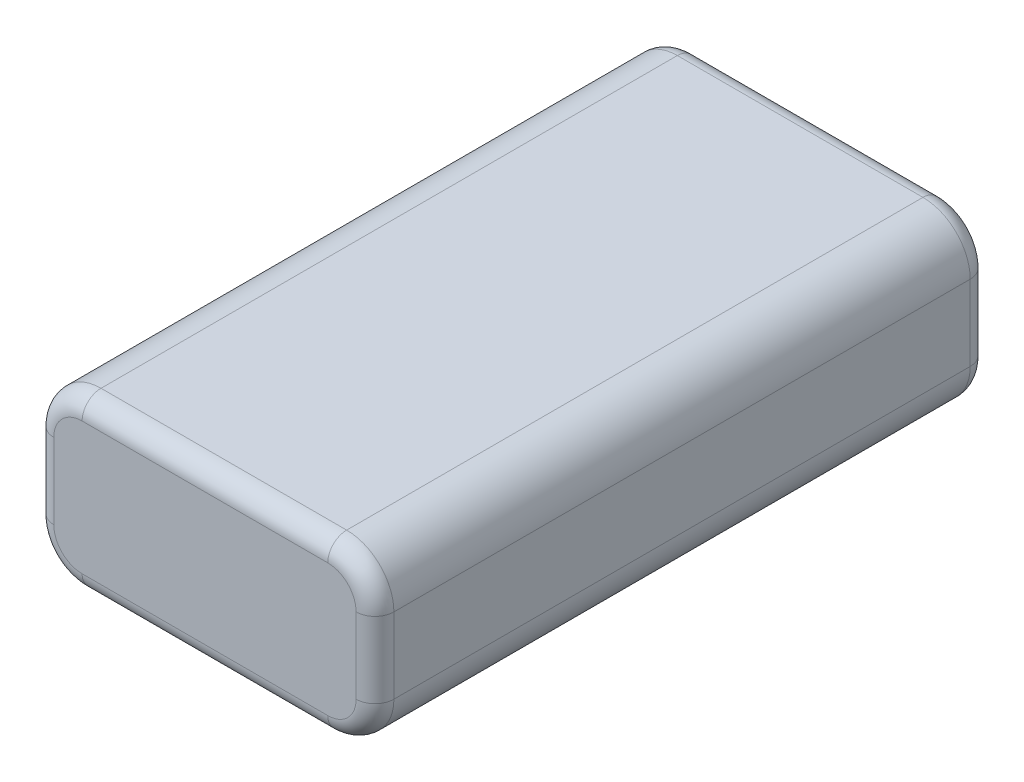
SolidWorks part; units mm, degrees
ref_plane "Front Plane" through (0, 0, 0) normal (0, 0, 1) x (1, 0, 0)
ref_plane "Top Plane" through (0, 0, 0) normal (0, 1, 0) x (1, 0, 0)
ref_plane "Right Plane" through (0, 0, 0) normal (1, 0, 0) x (0, 0, -1)
sketch "Sketch1" plane through (0, 0, 0) normal (0, 0, 1) x (1, 0, 0)
  line L1 (-18, 9) -> (18, 9)
  line L2 (-18, 9) -> (-18, -9)
  line L3 (-18, -9) -> (18, -9)
  line L4 (18, 9) -> (18, -9)
  line L5 (-18, 9) -> (18, -9) construction
  line L6 (-18, -9) -> (18, 9) construction
  point P0 (0, 0)
  dimension "D1" = 36
  dimension "D2" = 18
extrude "Boss-Extrude1" add sketch "Sketch1" along normal blind 65
fillet "Fillet1" radius 5 4 edges at (-18, -9, 32.5) (-18, 9, 32.5) (18, -9, 32.5) (18, 9, 32.5)
fillet "Fillet2" radius 2 16 edges at (16.5355, -7.5355, 0) (18, 0, 0) (16.5355, 7.5355, 0) (0, 9, 0) (-16.5355, 7.5355, 0) (-18, 0, 0) (-16.5355, -7.5355, 0) (0, -9, 0) (-16.5355, 7.5355, 65) (0, 9, 65) (16.5355, 7.5355, 65) (18, 0, 65) (16.5355, -7.5355, 65) (0, -9, 65) (-16.5355, -7.5355, 65) (-18, 0, 65)
